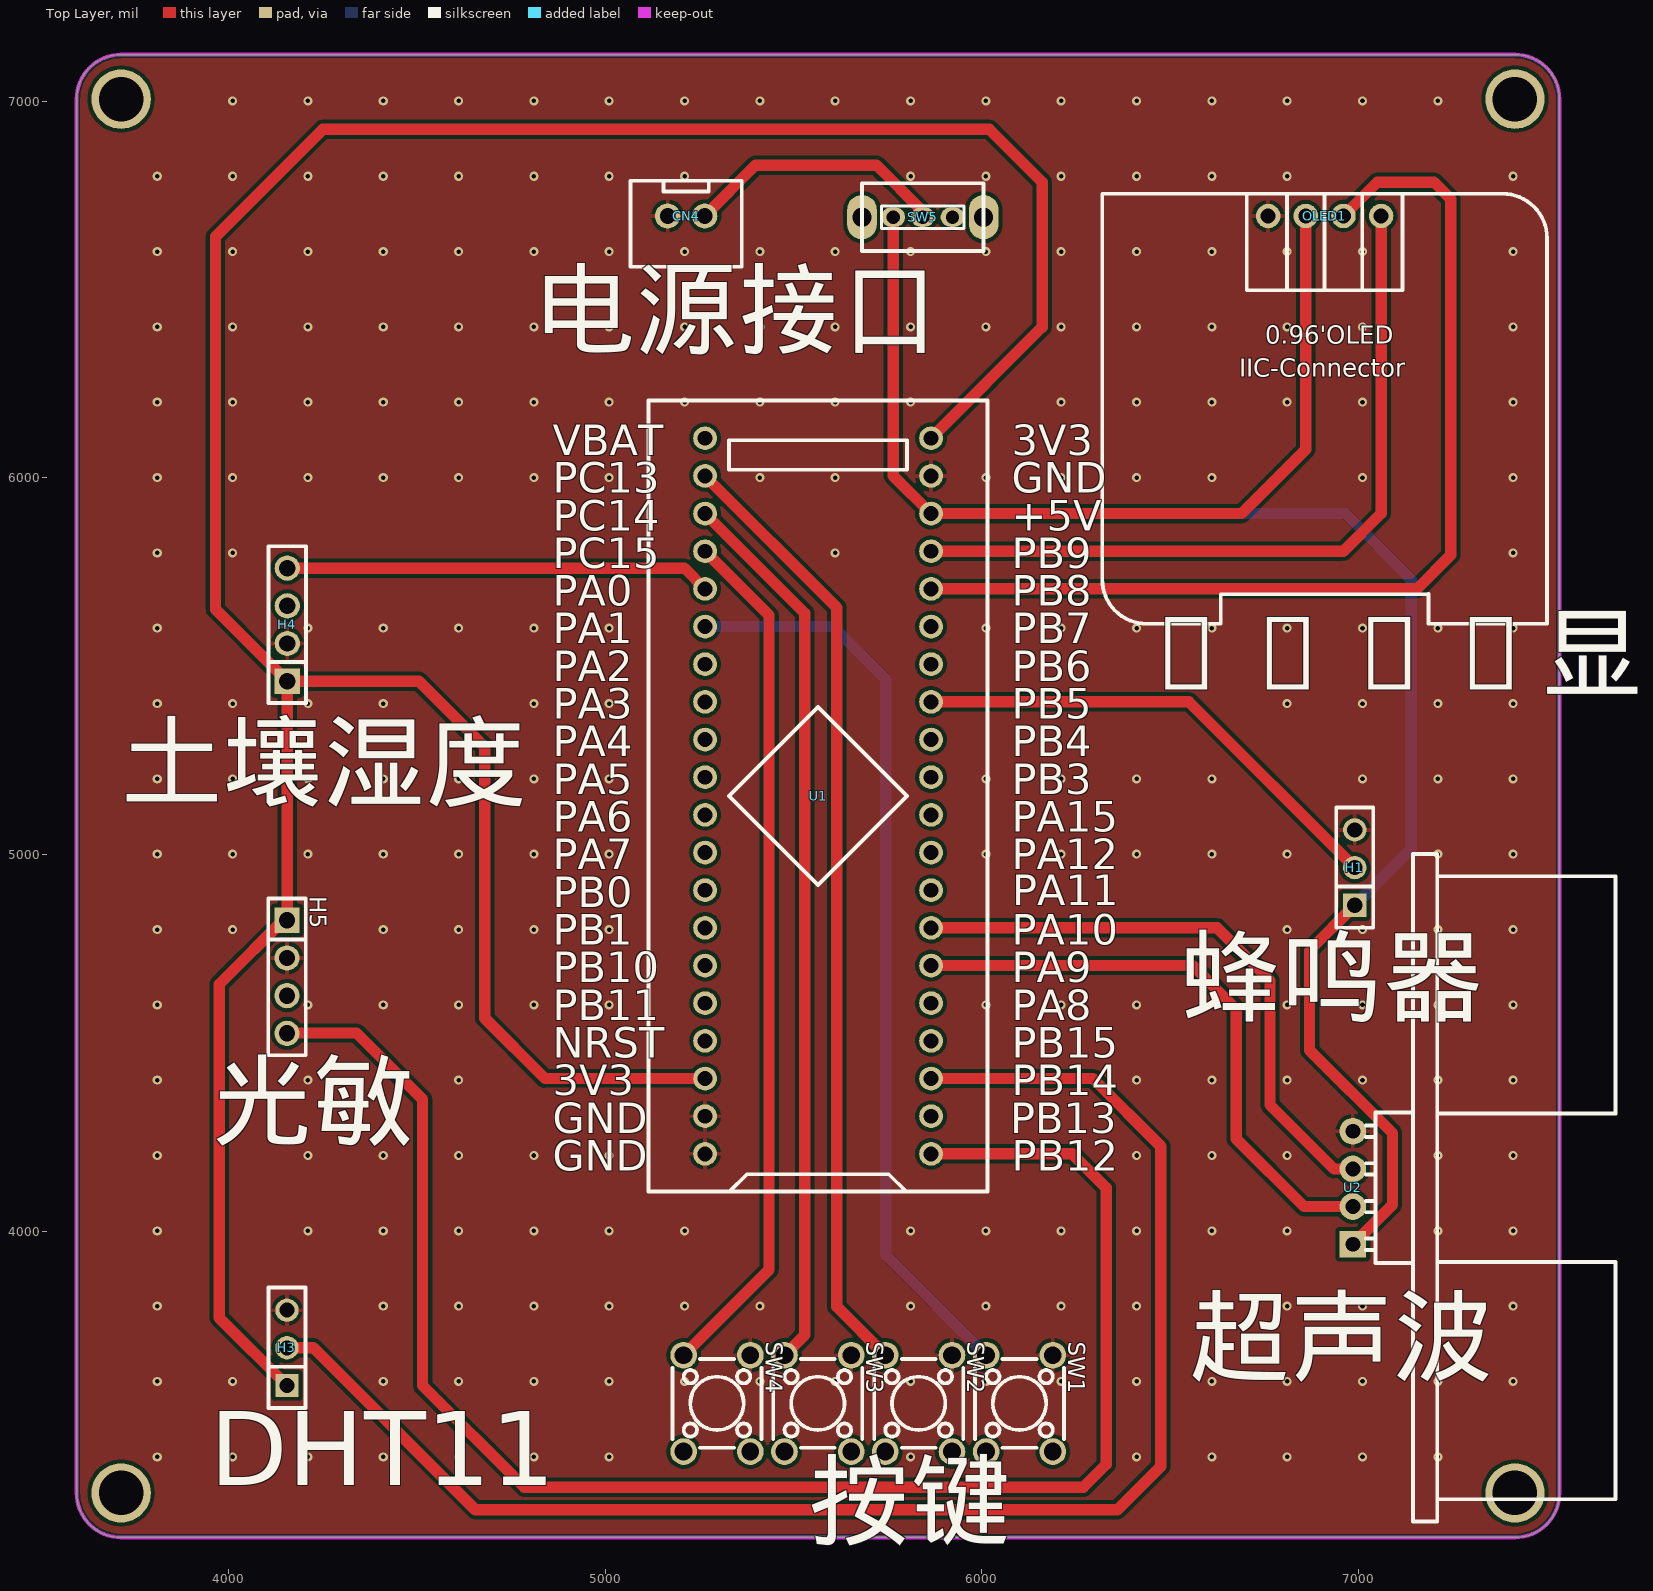
[diagram p0: Top Layer view]
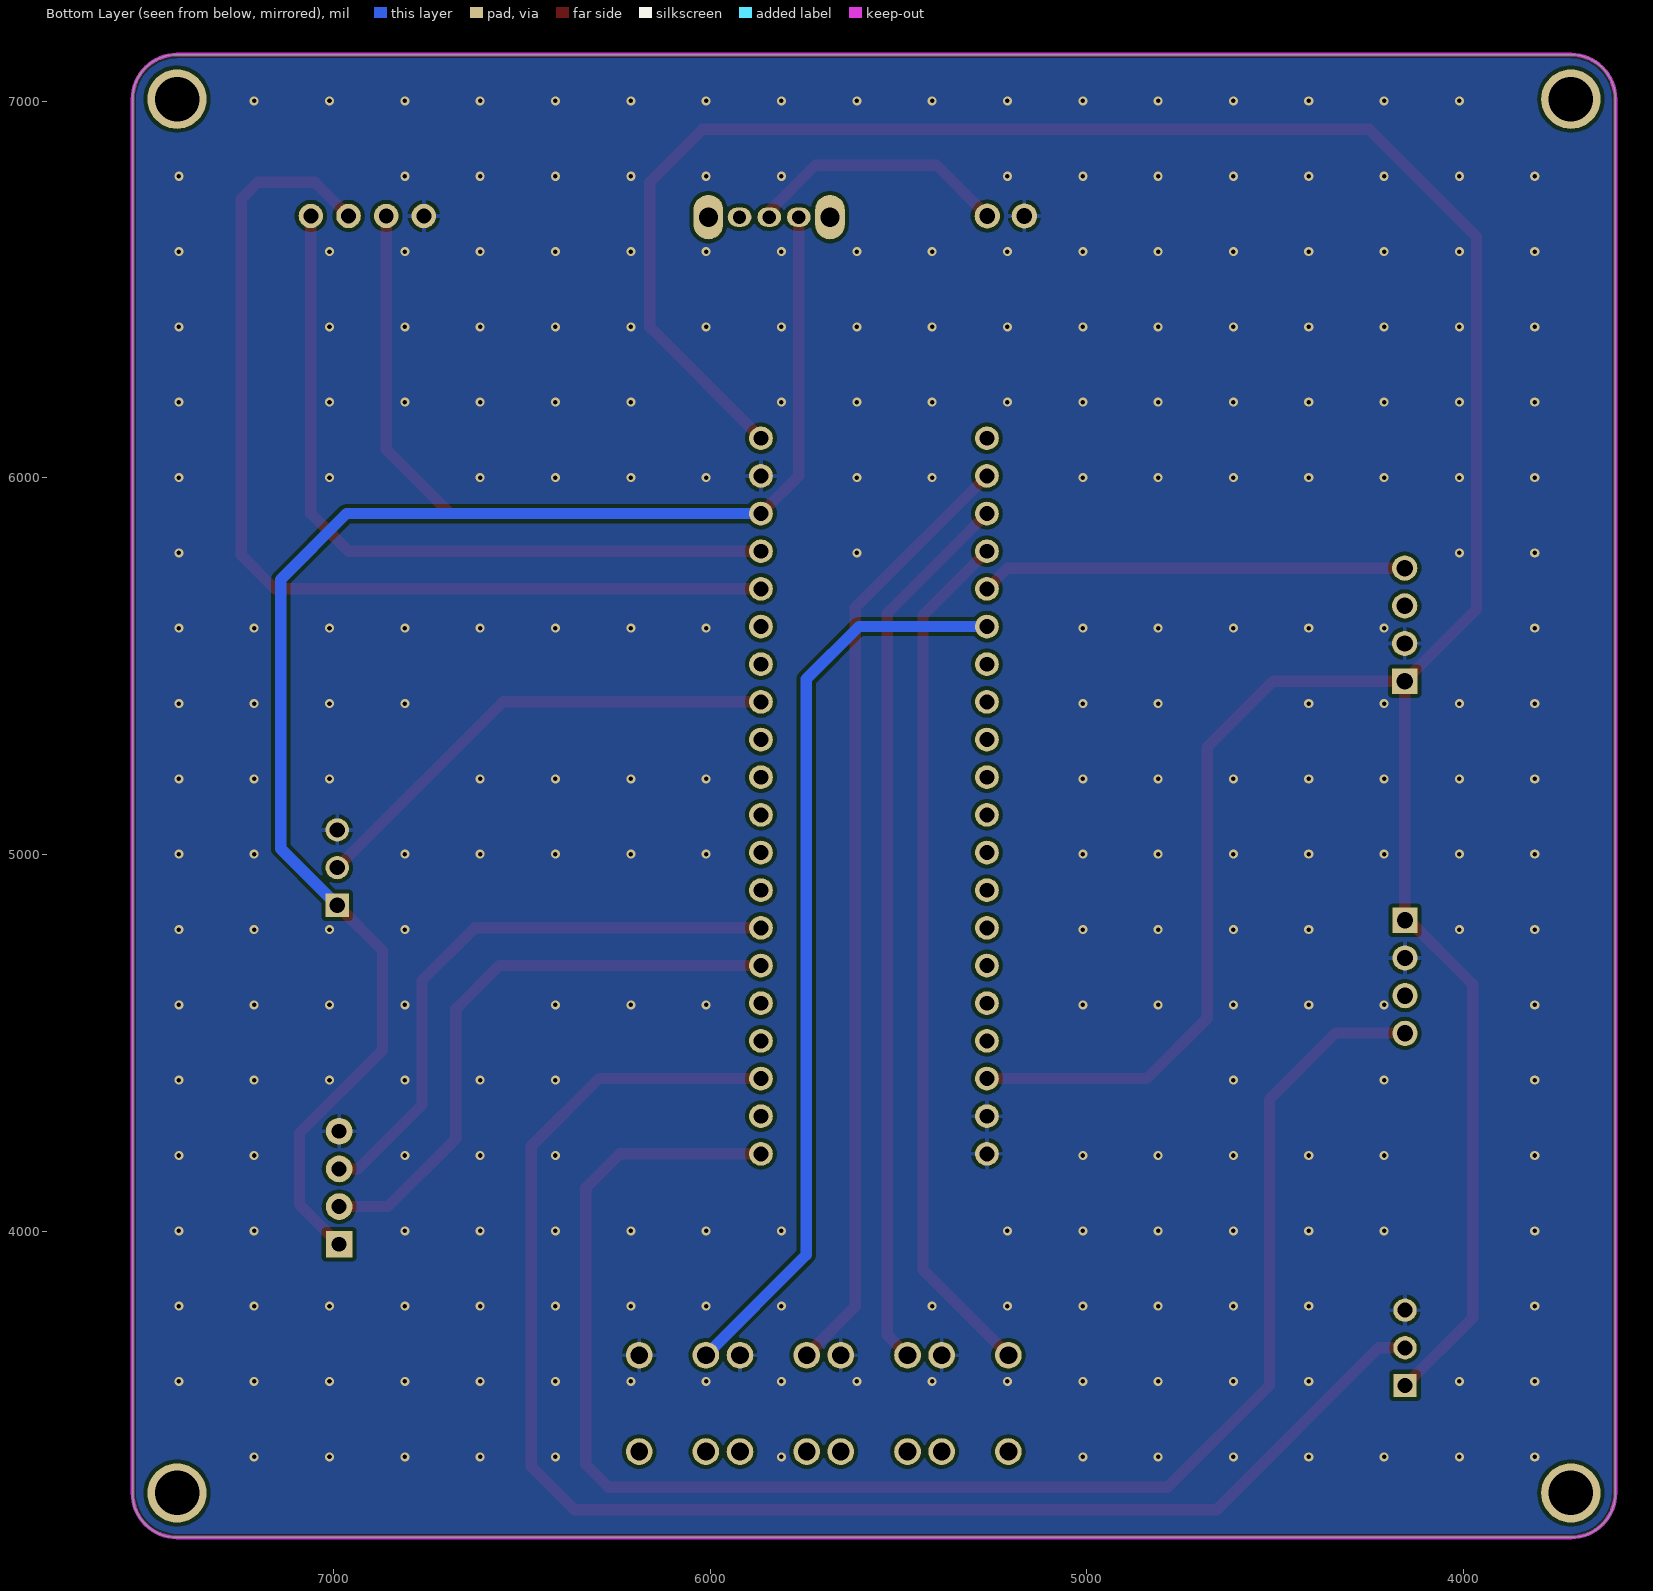
[diagram p1: Bottom Layer view, seen from below]
# Altium PCB MISC51673.pcbdoc
Units mil, origin at the board's own origin, x right, y up, seen from the top; angles counter-clockwise.
Board outline 3937.01 x 3937.01 mil, 2 copper layers (Top Layer, Bottom Layer), stack 62.206 mil thick; 13 components, 38 nets, 89 pads, 261 vias.

## Layer stack, top to bottom
Top Solder Mask Layer: solder mask 0.394, Dk 3.3
Top Layer: signal copper 1.379
Dielectric1: surface 59.449, FR4, Dk 4.5
Bottom Layer: signal copper 1.378
Bottom Solder Mask Layer: solder mask 0.394, Dk 3.3

## Board outline
3714.61,7123.5 ccw(c3714.61,7005.39) 3596.5,7005.39 3596.5,3304.61 ccw(c3714.61,3304.61) 3714.61,3186.5 7415.39,3186.5 ccw(c7415.39,3304.61) 7533.5,3304.61 7533.5,7005.39 ccw(c7415.39,7005.39) 7415.39,7123.5 3714.61,7123.5

## Design rules (kind name [scope] priority, off if disabled: settings)
BoardOutlineClearance copperThickness2oz_1 [All] p2 off: genericclearance=7.99 ignorepadtopadclearanceinfootprint=FALSE except(0: Arc-SplitContinuation Track-SplitContinuation SMDPad-SplitContinuation THPad-SplitContinuation Via-SplitContinuation Fill-SplitContinuation Region-SplitContinuation Poly-SplitContinuation Text-SplitContinuation Hole-SplitContinuation; 5.98: Arc-CutoutEdge Track-CutoutEdge SMDPad-CutoutEdge THPad-CutoutEdge Via-CutoutEdge Text-CutoutEdge; 6.9: Hole-OutlineEdge Hole-CutoutEdge; 10: Poly-OutlineEdge Poly-CutoutEdge; 11.81: Arc-OutlineEdge Track-OutlineEdge SMDPad-OutlineEdge THPad-OutlineEdge Via-OutlineEdge Fill-OutlineEdge Region-OutlineEdge Text-OutlineEdge Fill-CutoutEdge Region-CutoutEdge)
BoardOutlineClearance Plane_innerPlane_1 [All] p4 off: genericclearance=4.02 ignorepadtopadclearanceinfootprint=FALSE except(0: Arc-SplitContinuation Track-SplitContinuation SMDPad-SplitContinuation THPad-SplitContinuation Via-SplitContinuation Fill-SplitContinuation Region-SplitContinuation Poly-SplitContinuation Text-SplitContinuation Hole-SplitContinuation; 5.98: Arc-CutoutEdge Track-CutoutEdge SMDPad-CutoutEdge THPad-CutoutEdge Via-CutoutEdge Text-CutoutEdge; 6.9: Hole-OutlineEdge Hole-CutoutEdge; 10: Poly-OutlineEdge Poly-CutoutEdge; 11.81: Arc-OutlineEdge Track-OutlineEdge SMDPad-OutlineEdge THPad-OutlineEdge Via-OutlineEdge Fill-OutlineEdge Region-OutlineEdge Text-OutlineEdge Fill-CutoutEdge Region-CutoutEdge)
BoardOutlineClearance Copper_copperRegion_1 [All] p6 off: genericclearance=4.02 ignorepadtopadclearanceinfootprint=FALSE except(0: Arc-SplitContinuation Track-SplitContinuation SMDPad-SplitContinuation THPad-SplitContinuation Via-SplitContinuation Fill-SplitContinuation Region-SplitContinuation Poly-SplitContinuation Text-SplitContinuation Hole-SplitContinuation; 5.98: Arc-CutoutEdge Track-CutoutEdge SMDPad-CutoutEdge THPad-CutoutEdge Via-CutoutEdge Text-CutoutEdge; 6.9: Hole-OutlineEdge Hole-CutoutEdge; 10: Poly-OutlineEdge Poly-CutoutEdge; 11.81: Arc-OutlineEdge Track-OutlineEdge SMDPad-OutlineEdge THPad-OutlineEdge Via-OutlineEdge Fill-OutlineEdge Region-OutlineEdge Text-OutlineEdge Fill-CutoutEdge Region-CutoutEdge)
BoardOutlineClearance copperThickness1oz_1 [All] p8: genericclearance=4.02 ignorepadtopadclearanceinfootprint=FALSE except(0: Arc-SplitContinuation Track-SplitContinuation SMDPad-SplitContinuation THPad-SplitContinuation Via-SplitContinuation Fill-SplitContinuation Region-SplitContinuation Poly-SplitContinuation Text-SplitContinuation Hole-SplitContinuation; 5.98: Arc-CutoutEdge Track-CutoutEdge SMDPad-CutoutEdge THPad-CutoutEdge Via-CutoutEdge Text-CutoutEdge; 6.9: Hole-OutlineEdge Hole-CutoutEdge; 10: Poly-OutlineEdge Poly-CutoutEdge; 11.81: Arc-OutlineEdge Track-OutlineEdge SMDPad-OutlineEdge THPad-OutlineEdge Via-OutlineEdge Fill-OutlineEdge Region-OutlineEdge Text-OutlineEdge Fill-CutoutEdge Region-CutoutEdge)
Clearance copperThickness2oz [All] p1 off: gap=7.99 ignorepadtopadclearanceinfootprint=FALSE except(5.98: SMDPad-Track SMDPad-SMDPad THPad-Track SMDPad-THPad THPad-THPad Track-Via SMDPad-Via THPad-Via Via-Via Fill-SMDPad Region-SMDPad Fill-THPad Region-THPad Fill-Via Region-Via Fill-Fill Fill-Region Region-Region Arc-Track Arc-SMDPad Arc-THPad Arc-Via Fill-Arc Region-Arc Arc-Arc Text-Track SMDPad-Text Text-THPad Text-Via Fill-Text Region-Text Arc-Text Text-Text; 6.9: Hole-Track Hole-SMDPad Hole-THPad Hole-Via Fill-Hole Region-Hole Hole-Arc Hole-Text; 10: Poly-Track Poly-SMDPad Poly-THPad Poly-Via Poly-Fill Poly-Region Poly-Poly Poly-Arc Poly-Text Poly-Hole; 11.81: Fill-Track Region-Track)
Clearance Plane_innerPlane [All] p3 off: gap=4.02 ignorepadtopadclearanceinfootprint=FALSE except(5.98: SMDPad-Track SMDPad-SMDPad THPad-Track SMDPad-THPad THPad-THPad Track-Via SMDPad-Via THPad-Via Via-Via Fill-SMDPad Region-SMDPad Fill-THPad Region-THPad Fill-Via Region-Via Fill-Fill Fill-Region Region-Region Arc-Track Arc-SMDPad Arc-THPad Arc-Via Fill-Arc Region-Arc Arc-Arc Text-Track SMDPad-Text Text-THPad Text-Via Fill-Text Region-Text Arc-Text Text-Text; 6.9: Hole-Track Hole-SMDPad Hole-THPad Hole-Via Fill-Hole Region-Hole Hole-Arc Hole-Text; 10: Poly-Track Poly-SMDPad Poly-THPad Poly-Via Poly-Fill Poly-Region Poly-Poly Poly-Arc Poly-Text Poly-Hole; 11.81: Fill-Track Region-Track)
Clearance Copper_copperRegion [All] p5 off: gap=4.02 ignorepadtopadclearanceinfootprint=FALSE except(5.98: SMDPad-Track SMDPad-SMDPad THPad-Track SMDPad-THPad THPad-THPad Track-Via SMDPad-Via THPad-Via Via-Via Fill-SMDPad Region-SMDPad Fill-THPad Region-THPad Fill-Via Region-Via Fill-Fill Fill-Region Region-Region Arc-Track Arc-SMDPad Arc-THPad Arc-Via Fill-Arc Region-Arc Arc-Arc Text-Track SMDPad-Text Text-THPad Text-Via Fill-Text Region-Text Arc-Text Text-Text; 6.9: Hole-Track Hole-SMDPad Hole-THPad Hole-Via Fill-Hole Region-Hole Hole-Arc Hole-Text; 10: Poly-Track Poly-SMDPad Poly-THPad Poly-Via Poly-Fill Poly-Region Poly-Poly Poly-Arc Poly-Text Poly-Hole; 11.81: Fill-Track Region-Track)
Clearance copperThickness1oz [All] p7: gap=4.02 ignorepadtopadclearanceinfootprint=FALSE except(5.98: SMDPad-Track SMDPad-SMDPad THPad-Track SMDPad-THPad THPad-THPad Track-Via SMDPad-Via THPad-Via Via-Via Fill-SMDPad Region-SMDPad Fill-THPad Region-THPad Fill-Via Region-Via Fill-Fill Fill-Region Region-Region Arc-Track Arc-SMDPad Arc-THPad Arc-Via Fill-Arc Region-Arc Arc-Arc Text-Track SMDPad-Text Text-THPad Text-Via Fill-Text Region-Text Arc-Text Text-Text; 6.9: Hole-Track Hole-SMDPad Hole-THPad Hole-Via Fill-Hole Region-Hole Hole-Arc Hole-Text; 10: Poly-Track Poly-SMDPad Poly-THPad Poly-Via Poly-Fill Poly-Region Poly-Poly Poly-Arc Poly-Text Poly-Hole; 11.81: Fill-Track Region-Track)
DiffPairsRouting differentialPair [All] p1: maxlimit=6 minlimit=6 mostfreqgap=6 toplayer_minwidth=5 toplayer_prefwidth=10 toplayer_maxwidth=100 toplayer_mingap=6 toplayer_prefgap=6 toplayer_maxgap=6 bottomlayer_minwidth=5 bottomlayer_prefwidth=10 bottomlayer_maxwidth=100 bottomlayer_mingap=6 bottomlayer_prefgap=6 bottomlayer_maxgap=6 maxuncoupledlength=10
HoleToHoleClearance otherClearance [All] p1: gap=11.81 allowstackedmicrovias=TRUE
Length netLength [All] p1: minlimit=0 maxlimit=0
PasteMaskExpansion pasteMaskExpansion [All] p1: expansion=0
PlaneConnect innerPlane [All] p1: planeconnectstyle=Relief reliefexpansion=20 reliefentries=4 reliefconductorwidth=10 reliefairgap=10
PolygonConnect copperRegion [All] p1: connectstyle=Relief reliefconductorwidth=10 reliefentries=4 polygonreliefangle="90 Angle" airgapwidth=10 via.connectstyle=Relief via.reliefconductorwidth=10 via.reliefentries=4 via.polygonreliefangle="90 Angle" via.airgapwidth=10
RoutingVias viaSize [All] p1: holewidth=12.01 width=24.02 viastyle="Through Hole" minholewidth=11.81 minwidth=19.68 maxholewidth=248.03 maxwidth=393.7
SolderMaskExpansion solderMaskExpansion [IsVia] p1: expansion=-1000 istentingtop=TRUE
SolderMaskExpansion solderMaskExpansion [All] p2: expansion=2 istentingtop=FALSE
Width copperThickness2oz_2 [All] p1 off: maxlimit=100 minlimit=8 preferedwidth=10
Width copperThickness1oz_2 [All] p2: maxlimit=100 minlimit=5 preferedwidth=10

## Components (designator, comment, footprint, x,y, rotation, side; value= is the part's Value field where it differs from the comment)
CN4 "XH2.54*2P_直插" CONN-TH_2P-P2.50-XH2.54-2P 5215,6695 r0 top
H1 "" HDR-TH_3P-P2.54-V-F 6990,4965 r90 top
H3 "" HDR-TH_3P-P2.54-V-F 4155,3690 r90 top
H4 "" HDR-TH_4P-P2.54-V-F 4155.79,5610 r90 top
H5 "" HDR-TH_4P-P2.54-V-F 4155,4675 r270 top
OLED1 "" 0.96OLED_4P 6910,6695 r0 top
SW1 "" SW-TH_4P-L6.0-W6.0-P4.50-LS6.5 6099.85,3542.47 r270 top
SW2 "" SW-TH_4P-L6.0-W6.0-P4.50-LS6.5 5832.14,3542.47 r270 top
SW3 "" SW-TH_4P-L6.0-W6.0-P4.50-LS6.5 5564.43,3542.47 r270 top
SW4 "" SW-TH_4P-L6.0-W6.0-P4.50-LS6.5 5296.72,3542.47 r270 top
SW5 "" 拨动开关 5837.9,6692.05 r0 top
U1 "STM32F103C8T6-Card" CONN-TH_L53.3-W22.9_STM32F103C8T6-CARD 5565,5155 r90 top
U2 "HC-SR04" TH_HC-SR04V 6985,4115 r90 top

## Footprints (in the part's own frame and the unit in brackets; to place one, negate y for a bottom-side part, rotate by r counter-clockwise, add the part's x,y. Pads: shape width x height; smd on the part's side, far side on the other; paste and mask are expansions set on the pad)
0.96OLED_4P [mm]
  round 1.65 hole 1 copper offset 0,0: 1(-3.81,-0.001) 2(-1.27,0.002) 3(1.27,0.002) 4(3.81,0.002)
  silkscreen extent -15,-27.5 15,1.5
CONN-TH_2P-P2.50-XH2.54-2P [mm]
  round 1.7 hole 1.05 paste+0 mask+0.05: 1(1.25,0) 2(-1.25,0)
  silkscreen extent -3.75,-3.42 3.75,2.37
CONN-TH_L53.3-W22.9_STM32F103C8T6-CARD [mm]
  round 1.6 hole 1: 1(-24.13,-7.62) 2(-21.59,-7.62) 3(-19.05,-7.62) 4(-16.51,-7.62) 5(-13.97,-7.62) 6(-11.43,-7.62) 7(-8.89,-7.62) 8(-6.35,-7.62) 9(-3.81,-7.62) 10(-1.27,-7.62) 11(1.27,-7.62) 12(3.81,-7.62) 13(6.35,-7.62) 14(8.89,-7.62) 15(11.43,-7.62) 16(13.97,-7.62) 17(16.51,-7.62) 18(19.05,-7.62) 19(21.59,-7.62) 20(24.13,-7.62) 21(24.13,7.62) 22(21.59,7.62) 23(19.05,7.62) 24(16.51,7.62) 25(13.97,7.62) 26(11.43,7.62) 27(8.89,7.62) 28(6.35,7.62) 29(3.81,7.62) 30(1.27,7.62) 31(-1.27,7.62) 32(-3.81,7.62) 33(-6.35,7.62) 34(-8.89,7.62) 35(-11.43,7.62) 36(-13.97,7.62) 37(-16.51,7.62) 38(-19.05,7.62) 39(-21.59,7.62) 40(-24.13,7.62)
  silkscreen extent -26.67,-11.43 26.67,11.43
HDR-TH_3P-P2.54-V-F [mil]
  rect 62x62 hole 40.16: 1(-100,0)
  round 62 hole 40.16: 2(0,0) 3(100,0)
  silkscreen extent -160,-49 160,49
HDR-TH_4P-P2.54-V-F [mm]
  rect 1.7x1.7 hole 1.1: 1(-3.81,0)
  round 1.7 hole 1.1: 2(-1.27,0) 3(1.27,0) 4(3.81,0)
  silkscreen extent -5.29,-1.27 5.29,1.27
SW-TH_4P-L6.0-W6.0-P4.50-LS6.5 [mm]
  round 1.8 hole 1.2: 1(-3.25,2.25) 2(3.25,2.25) 3(-3.25,-2.25) 4(3.25,-2.25)
  silkscreen extent -3,-3 3,3
TH_HC-SR04V [mm]
  rect 1.8x1.8 hole 1.001: 1(-3.81,0)
  round 1.8 hole 1.001: 2(-1.27,0) 3(1.27,0) 4(3.81,0)
  silkscreen extent -22.5,-17.7 22.5,-0.89
拨动开关 [mil]
  oval 63x51.2 hole 35.4 paste+0 mask+2: 1(-73.4,0) 2(5,0) 3(84,0)
  oval 78.7x118.1 hole 51.2 paste+0 mask+2: 4(166.7,0) 5(-156.1,0)
  silkscreen extent -156,-90 167,90

## Free pads (board coordinates)
  round 157.48 hole 118.11: 1(3714.61,7005.39) 1(3714.61,3304.61) 1(7415.39,7005.39) 1(7415.39,3304.61)

## Via types
v1: diameter 24.02, hole 12, Top Layer to Bottom Layer, 261 vias

## Nets (pads, with @x,y where several pads share a name; then routed paths per layer and width w, separated by ;. In a path a pad name is that pad's centre, name@x,y a point inside that pad or via, vN(x,y) a via of type N, cw(c..) or ccw(c..) an arc to the next point about the centre after c; other vN are vias at no path point)
$1N17118: CN4.1 SW5.2 | length 700.6
  Top Layer w30: CN4.1 5399.22,6830 5720,6830 5842.9,6707.1 SW5.2
+5V: H1.1 OLED1.2 SW5.1 U1.18 U2.1 | length 5873.1
  Top Layer w30: SW5.1 5764.5,6005.5 U1.18 6690,5905 6860,6075 OLED1.2@6860,6695.05 ; U2.1 7090,4070 7090,4260 6870,4480 6870,4745 H1.1
  Bottom Layer w30: U1.18 6965,5905 7140,5730 7140,5015 H1.1
GND: CN4.2 H1.3 H3.3 H4.2 H5.2 OLED1.1 SW1.1 SW2.1 SW3.1 SW4.1 U1.19 U1.39 U1.40 U2.4
  other v1: 3810.6,3400.6 4010.6,3400.6 4210.6,3400.6 4410.6,3400.6 4610.6,3400.6 4810.6,3400.6 5010.6,3400.6 5810.6,3400.6 6410.6,3400.6 6610.6,3400.6 6810.6,3400.6 7010.6,3400.6 7210.6,3400.6 3810.6,3600.6 4010.6,3600.6 4410.6,3600.6 4610.6,3600.6 4810.6,3600.6 5010.6,3600.6 5210.6,3600.6 5410.6,3600.6 5610.6,3600.6 5810.6,3600.6 6010.6,3600.6 6210.6,3600.6 6410.6,3600.6 6610.6,3600.6 6810.6,3600.6 7010.6,3600.6 7210.6,3600.6 7410.6,3600.6 3810.6,3800.6 4410.6,3800.6 4610.6,3800.6 4810.6,3800.6 5010.6,3800.6 5210.6,3800.6 5410.6,3800.6 5810.6,3800.6 6010.6,3800.6 6210.6,3800.6 6410.6,3800.6 6610.6,3800.6 6810.6,3800.6 7010.6,3800.6 7210.6,3800.6 7410.6,3800.6 3810.6,4000.6 4210.6,4000.6 4410.6,4000.6 4610.6,4000.6 4810.6,4000.6 5010.6,4000.6 5210.6,4000.6 5810.6,4000.6 6010.6,4000.6 6210.6,4000.6 6410.6,4000.6 6610.6,4000.6 6810.6,4000.6 7210.6,4000.6 7410.6,4000.6 3810.6,4200.6 4210.6,4200.6 4410.6,4200.6 4610.6,4200.6 4810.6,4200.6 5010.6,4200.6 6410.6,4200.6 6610.6,4200.6 6810.6,4200.6 7210.6,4200.6 7410.6,4200.6 3810.6,4400.6 4210.6,4400.6 4610.6,4400.6 6410.6,4400.6 6610.6,4400.6 6810.6,4400.6 7010.6,4400.6 7210.6,4400.6 7410.6,4400.6 3810.6,4600.6 4210.6,4600.6 4410.6,4600.6 4610.6,4600.6 4810.6,4600.6 5010.6,4600.6 6010.6,4600.6 6210.6,4600.6 6410.6,4600.6 6810.6,4600.6 7010.6,4600.6 7210.6,4600.6 7410.6,4600.6 3810.6,4800.6 4010.6,4800.6 4410.6,4800.6 4610.6,4800.6 4810.6,4800.6 5010.6,4800.6 6810.6,4800.6 7010.6,4800.6 7210.6,4800.6 7410.6,4800.6 3810.6,5000.6 4010.6,5000.6 4210.6,5000.6 4410.6,5000.6 4610.6,5000.6 4810.6,5000.6 5010.6,5000.6 6010.6,5000.6 6210.6,5000.6 6410.6,5000.6 6610.6,5000.6 6810.6,5000.6 7210.6,5000.6 7410.6,5000.6 3810.6,5200.6 4010.6,5200.6 4210.6,5200.6 4410.6,5200.6 4610.6,5200.6 4810.6,5200.6 5010.6,5200.6 6010.6,5200.6 6210.6,5200.6 6410.6,5200.6 6610.6,5200.6 7010.6,5200.6 7210.6,5200.6 7410.6,5200.6 3810.6,5400.6 4010.6,5400.6 4210.6,5400.6 4410.6,5400.6 4810.6,5400.6 5010.6,5400.6 6810.6,5400.6 7010.6,5400.6 7210.6,5400.6 7410.6,5400.6 3810.6,5600.6 4210.6,5600.6 4410.6,5600.6 4610.6,5600.6 4810.6,5600.6 5010.6,5600.6 6010.6,5600.6 6210.6,5600.6 6410.6,5600.6 6610.6,5600.6 6810.6,5600.6 7010.6,5600.6 7210.6,5600.6 7410.6,5600.6 3810.6,5800.6 4010.6,5800.6 5610.6,5800.6 7410.6,5800.6 3810.6,6000.6 4010.6,6000.6 4210.6,6000.6 4410.6,6000.6 4610.6,6000.6 4810.6,6000.6 5010.6,6000.6 5410.6,6000.6 5610.6,6000.6 6010.6,6000.6 6210.6,6000.6 6410.6,6000.6 6610.6,6000.6 7010.6,6000.6 7410.6,6000.6 3810.6,6200.6 4010.6,6200.6 4210.6,6200.6 4410.6,6200.6 4610.6,6200.6 4810.6,6200.6 5010.6,6200.6 5210.6,6200.6 5410.6,6200.6 5610.6,6200.6 5810.6,6200.6 6210.6,6200.6 6410.6,6200.6 6610.6,6200.6 6810.6,6200.6 7010.6,6200.6 7410.6,6200.6 3810.6,6400.6 4010.6,6400.6 4210.6,6400.6 4410.6,6400.6 4610.6,6400.6 4810.6,6400.6 5010.6,6400.6 5210.6,6400.6 5410.6,6400.6 5610.6,6400.6 5810.6,6400.6 6010.6,6400.6 6210.6,6400.6 6410.6,6400.6 6610.6,6400.6 6810.6,6400.6 7010.6,6400.6 7410.6,6400.6 3810.6,6600.6 4010.6,6600.6 4210.6,6600.6 4410.6,6600.6 4610.6,6600.6 4810.6,6600.6 5010.6,6600.6 5210.6,6600.6 5410.6,6600.6 5610.6,6600.6 5810.6,6600.6 6010.6,6600.6 6210.6,6600.6 6410.6,6600.6 6610.6,6600.6 6810.6,6600.6 7010.6,6600.6 7410.6,6600.6 3810.6,6800.6 4010.6,6800.6 4210.6,6800.6 4410.6,6800.6 4610.6,6800.6 4810.6,6800.6 5010.6,6800.6 5210.6,6800.6 5810.6,6800.6 6010.6,6800.6 6210.6,6800.6 6410.6,6800.6 6610.6,6800.6 6810.6,6800.6 7410.6,6800.6 4010.6,7000.6 4210.6,7000.6 4410.6,7000.6 4610.6,7000.6 4810.6,7000.6 5010.6,7000.6 5210.6,7000.6 5410.6,7000.6 5610.6,7000.6 5810.6,7000.6 6010.6,7000.6 6210.6,7000.6 6410.6,7000.6 6610.6,7000.6 6810.6,7000.6 7010.6,7000.6 7210.6,7000.6
NRST: U1.37
PA0: H4.4 U1.25 | length 1132
  Top Layer w30: H4.4 5210,5760 U1.25
PA1: SW1.3 U1.26 | length 2442.9
  Bottom Layer w30: U1.26 5605,5605 5745,5465 5745,3936.69 SW1.3
PA2: U1.27
PA3: U1.28
PA4: U1.29
PA5: U1.30
PA6: U1.31
PA7: U1.32
PA8: U1.5
PA9: U1.6 U2.2 | length 1587.2
  Top Layer w30: U1.6 6560,4705 6675,4590 6675,4245 6855,4065 U2.2
PA10: U1.7 U2.3 | length 1578.4
  Top Layer w30: U1.7 6625,4805 6765,4665 6765,4335 6935,4165 U2.3
PA11: U1.8
PA12: U1.9
PA15: U1.10
PB0: U1.33
PB1: U1.34
PB3: U1.11
PB4: U1.12
PB5: H1.2 U1.13 | length 1307.3
  Top Layer w30: U1.13 6550,5405 H1.2
PB6: U1.14
PB7: U1.15
PB8: OLED1.3 U1.16 | length 2703.2
  Top Layer w30: U1.16 7155,5705 7245,5795 7245,6740 7200,6785 7049.95,6785 OLED1.3@6960,6695.05
PB9: OLED1.4 U1.17 | length 2026.5
  Top Layer w30: U1.17 6960,5805 7060,5905 OLED1.4@7060,6695.05
PB10: U1.35
PB11: U1.36
PB12: H5.4 U1.1 | length 4381.8
  Top Layer w30: H5.4@4155,4525.79 4339.21,4525.79 4515,4350 4515,3590 4785,3320 6270,3320 6330,3380 6330,4115 6240,4205 U1.1
PB13: U1.2
PB14: H3.2 U1.3 | length 4080.3
  Top Layer w30: H3.2 4225,3690 4655,3260 6360,3260 6475,3375 6475,4225 6295,4405 U1.3
PB15: U1.4
PC13: SW2.3 U1.22 | length 2532.8
  Top Layer w30: U1.22 5615,5655 5615,3798.98 SW2.3
PC14: SW3.3 U1.23 | length 2366.8
  Top Layer w30: U1.23 5530,5640 5530,3724.57 SW3.3
PC15: SW4.3 U1.24 | length 2299
  Top Layer w30: SW4.3 5435,3897.28 5435,5635 U1.24
VBAT: U1.21
VCC: H3.1 H4.1 H5.1 U1.20 U1.38 | length 8419.7
  Top Layer w30: H3.1 3975,3770 3975,4655 4155.79,4835.79 H4.1 ; U1.38 4840,4405 4680,4565 4680,5285 4505,5460 H4.1 ; U1.20 6160,6400 6160,6785 6020,6925 4250,6925 3965,6640 3965,5650.79 H4.1
pads on no net: H4.3 H5.3 SW1.2 SW1.4 SW2.2 SW2.4 SW3.2 SW3.4 SW4.2 SW4.4 SW5.3 SW5.4 SW5.5

## Polygon pours and split planes (outlines as drawn)
GND on Bottom Layer (solid, remove dead copper, pour order 2): 3525,7245 3525,3080 7700,3080 7700,7245
GND on Top Layer (solid, remove dead copper, pour order 2): 3000,7415 3000,3000 7930,3000 7930,7415

## Keep-outs
Board Outline Layer:
  the board outline again, w10

## Silkscreen, mask and mechanical layers (free items; w line width, h text height)
Top Silkscreen Layer:
  text "电源接口" at 4812.87,6351.57 h196.85
  text "VBAT" at 4860.95,6060 h80
  text "3V3" at 6079.16,6060 h80
  text "PC13" at 4860.95,5960 h80
  text "GND" at 6079.16,5960 h80
  text "PC14" at 4860.95,5860 h80
  text "+5V" at 6079.16,5860 h80
  text "PC15" at 4860.95,5760 h80
  text "PB9" at 6079.16,5760 h80
  text "PA0" at 4860.95,5660 h80
  text "PB8" at 6079.16,5660 h80
  text "PA1" at 4860.95,5560 h80
  text "PB7" at 6079.16,5560 h80
  text "PA2" at 4860.95,5460 h80
  text "PB6" at 6079.16,5460 h80
  text "Oled显示器" at 6408.66,5436.57 h196.85
  text "PA3" at 4860.95,5360 h80
  text "PB5" at 6079.16,5360 h80
  text "PA4" at 4860.95,5260 h80
  text "PB4" at 6079.16,5260 h80
  text "PA5" at 4860.95,5160 h80
  text "PB3" at 6079.16,5160 h80
  text "土壤湿度" at 3715,5150 h196.85
  text "PA6" at 4860.95,5060 h80
  text "PA15" at 6079.16,5060 h80
  text "PA7" at 4860.95,4960 h80
  text "PA12" at 6079.16,4960 h80
  text "PA11" at 6080.95,4865 h80
  text "PB0" at 4860.95,4860 h80
  text "PB1" at 4860.95,4760 h80
  text "PA10" at 6079.16,4760 h80
  text "PB10" at 4860.95,4660 h80
  text "PA9" at 6079.16,4660 h80
  text "蜂鸣器" at 6525,4580 h196.85
  text "PB11" at 4860.95,4560 h80
  text "PA8" at 6079.16,4560 h80
  text "NRST" at 4860.95,4460 h80
  text "PB15" at 6079.16,4460 h80
  text "3V3" at 4860.95,4360 h80
  text "PB14" at 6079.16,4360 h80
  text "GND" at 4860.95,4260 h80
  text "PB13" at 6075.95,4260 h80
  text "光敏" at 3955,4250 h196.85
  text "GND" at 4860.95,4160 h80
  text "PB12" at 6079.16,4160 h80
  text "超声波" at 6550,3625 h196.85
  text "DHT11" at 3950,3325 h196.85
  text "按键" at 5540,3190 h196.85